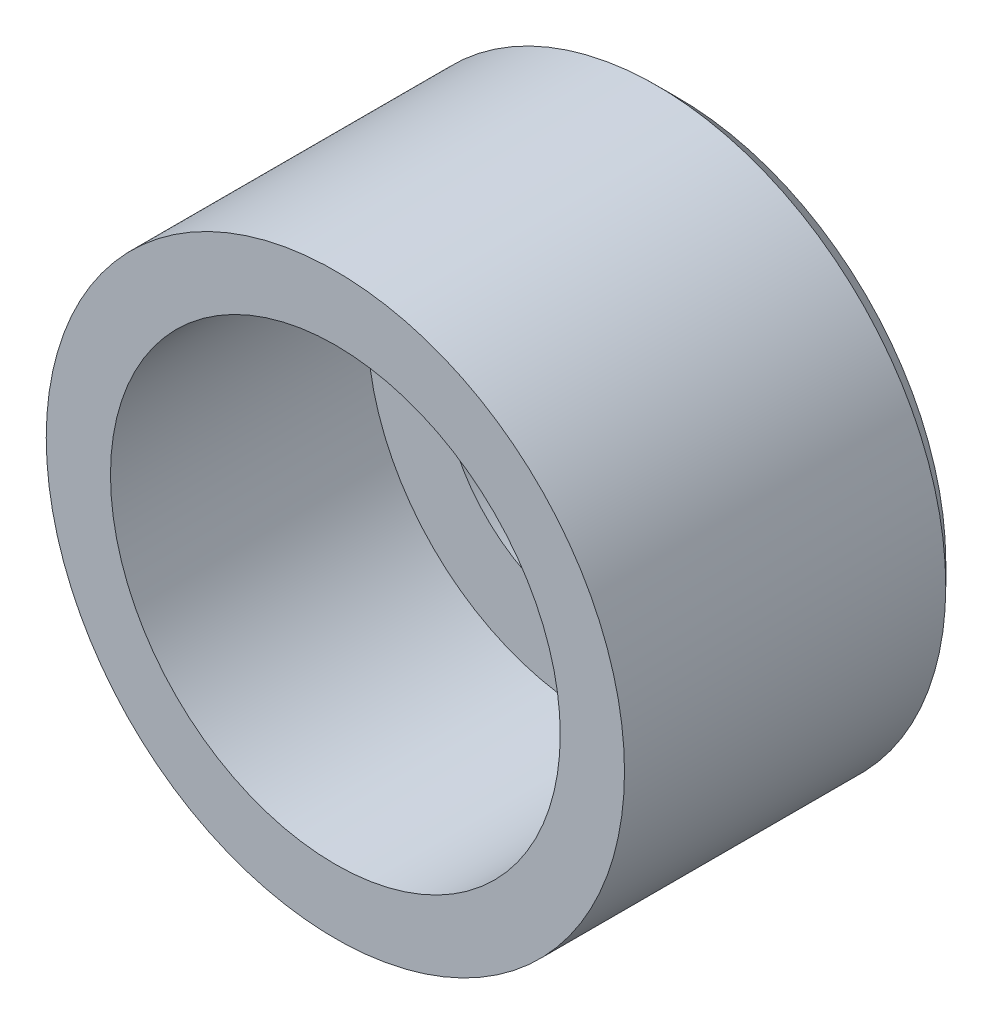
from build123d import *

# Parameters (mm, degrees)
SKETCH1_R           = 27
SKETCH1_R_2         = 14
BOSS_EXTRUDE1_DEPTH = 32
SKETCH2_R           = 21
CUT_EXTRUDE1_DEPTH  = 24
CHAMFER1_SIZE       = 2


with BuildPart() as part:
    # Sketch1 → Boss-Extrude1 (new body)
    with BuildSketch(Plane.XY):
        Circle(SKETCH1_R)
        Circle(SKETCH1_R_2, mode=Mode.SUBTRACT)
    extrude(amount=BOSS_EXTRUDE1_DEPTH)

    # Sketch2 → Cut-Extrude1 (cut)
    with BuildSketch(Plane.XY.offset(32)):
        Circle(SKETCH2_R)
    extrude(amount=-CUT_EXTRUDE1_DEPTH, mode=Mode.SUBTRACT)

    # Chamfer1
    chamfer1_edges = [part.edges().sort_by_distance(p)[0] for p in [
        (-27, 0, 0),
    ]]
    chamfer(chamfer1_edges, length=CHAMFER1_SIZE)


solid = part.part
